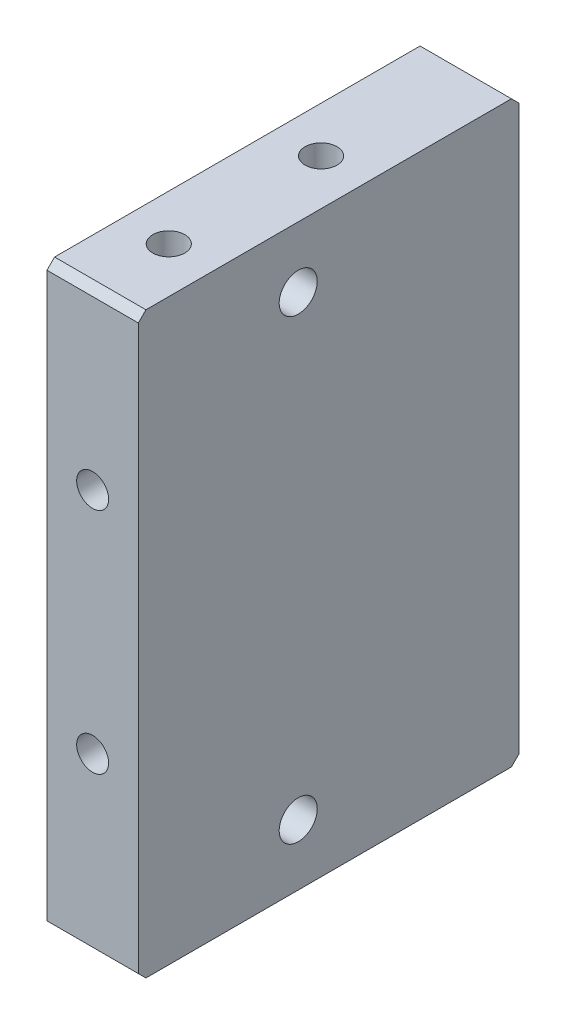
from build123d import *

# Parameters (mm, degrees)
SKETCH6_W                  = 50
SKETCH6_H                  = 76
BOSS_EXTRUDE6_DEPTH        = 12
M6_TAPPED_HOLE2_D          = 5
M6_TAPPED_HOLE2_DEPTH      = 15
M6_TAPPED_HOLE2_TIP        = 1.502151548
M5_TAPPED_HOLE3_AT_2_COUNT = 2
M5_TAPPED_HOLE3_AT_2_PITCH = 20
M5_TAPPED_HOLE2_D          = 4.2
M5_TAPPED_HOLE2_DEPTH      = 12.4
M5_TAPPED_HOLE2_TIP        = 1.2618073
CHAMFER1_SIZE              = 1


with BuildPart() as part:
    # Sketch6 → Boss-Extrude6 (new body)
    with BuildSketch(Plane(origin=(0, 0, 0), x_dir=(0, 0, -1), z_dir=(1, 0, 0))):
        with Locations((25, 0)):
            Rectangle(SKETCH6_W, SKETCH6_H)
    extrude(amount=-BOSS_EXTRUDE6_DEPTH)

    # M6 Tapped Hole2
    with Locations(Plane(origin=(0, 0, 0), x_dir=(0, 0, -1), z_dir=(1, 0, 0))):
        with Locations((21, -30), (21, 30)):
            Hole(M6_TAPPED_HOLE2_D / 2, depth=M6_TAPPED_HOLE2_DEPTH)
            with Locations((0, 0, -(M6_TAPPED_HOLE2_DEPTH + M6_TAPPED_HOLE2_TIP / 2))):  # 118° drill point
                Cone(0, M6_TAPPED_HOLE2_D / 2, M6_TAPPED_HOLE2_TIP, mode=Mode.SUBTRACT)

    # Sketch19 → M5 Tapped Hole3 (revolve, cut)
    with BuildSketch(Plane(origin=(-6, -38, -10), x_dir=(0, 0, -1), z_dir=(1, 0, 0))):
        Polygon((0, 0), (0, 18.6618073), (2.1, 17.4), (2.1, 0), align=None)
    m5_tapped_hole3 = revolve(axis=Axis((-6, -44.35, -10), (0, 1, 0)), mode=Mode.SUBTRACT)

    # M5 Tapped Hole3 at 2: M5 Tapped Hole3 ×2
    with Locations(*[(0, 0, -i * M5_TAPPED_HOLE3_AT_2_PITCH) for i in range(1, M5_TAPPED_HOLE3_AT_2_COUNT)]):
        add(m5_tapped_hole3, mode=Mode.SUBTRACT)

    # Mirror1: M5 Tapped Hole3 across plane
    add(m5_tapped_hole3.mirror(Plane.ZX), mode=Mode.SUBTRACT)

    # Mirror1 copy 1 sketch → Mirror1 copy 1 (revolve, cut)
    with BuildSketch(Plane(origin=(-6, 38, -30), x_dir=(0, 0, -1), z_dir=(1, 0, 0))):
        Polygon((0, 0), (0, -18.6618073), (2.1, -17.4), (2.1, 0), align=None)
    revolve(axis=Axis((-6, 44.35, -30), (0, 1, 0)), mode=Mode.SUBTRACT)

    # M5 Tapped Hole2
    with Locations(Plane.XY):
        with Locations((-6, 15), (-6, -15)):
            Hole(M5_TAPPED_HOLE2_D / 2, depth=M5_TAPPED_HOLE2_DEPTH)
            with Locations((0, 0, -(M5_TAPPED_HOLE2_DEPTH + M5_TAPPED_HOLE2_TIP / 2))):  # 118° drill point
                Cone(0, M5_TAPPED_HOLE2_D / 2, M5_TAPPED_HOLE2_TIP, mode=Mode.SUBTRACT)

    # Chamfer1
    chamfer1_edges = [part.edges().sort_by_distance(p)[0] for p in [
        (-6, 38, 0),
        (-6, 38, -50),
        (-6, -38, -50),
        (-6, -38, 0),
    ]]
    chamfer(chamfer1_edges, length=CHAMFER1_SIZE)


solid = part.part
